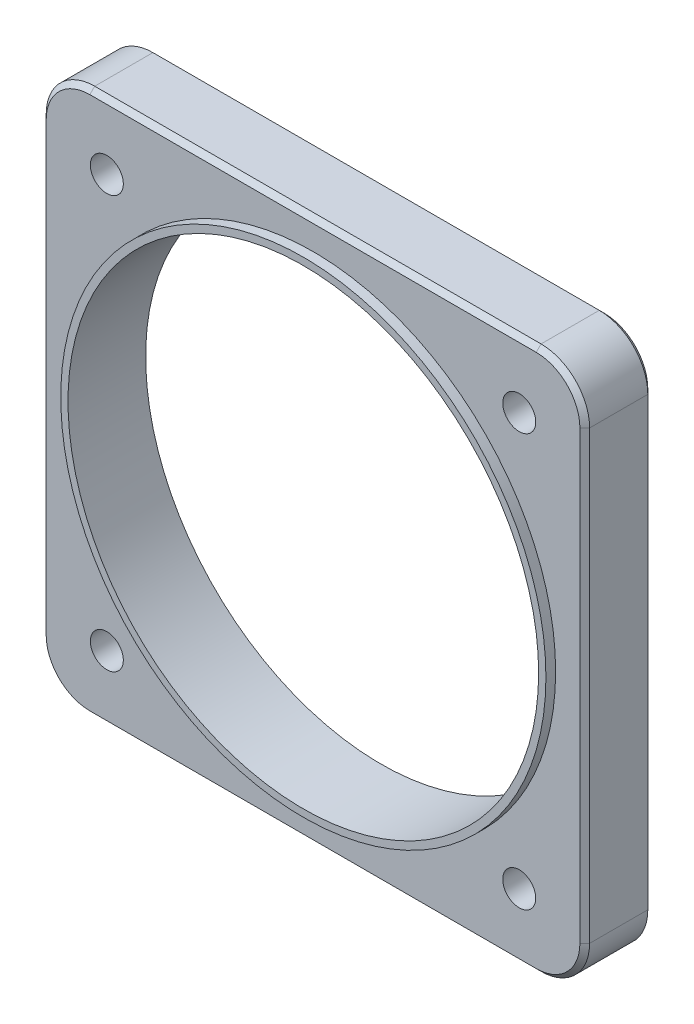
from build123d import *

# Parameters (mm, degrees)
SKETCH1_R           = 48.5
BOSS_EXTRUDE1_DEPTH = 16
SKETCH2_R           = 3.35
CUT_EXTRUDE1_DEPTH  = 81.796039507
M8_TAPPED_HOLE2_D   = 6.8
CUT_EXTRUDE2_START  = -2
SKETCH5_R           = 50
CUT_EXTRUDE2_DEPTH  = 2
CHAMFER1_SIZE       = 1


with BuildPart() as part:
    # Sketch1 → Boss-Extrude1 (new body)
    with BuildSketch(Plane.XY):
        with BuildLine():
            Line((-46, 56), (46, 56))
            ThreePointArc((46, 56), (53.071067812, 53.071067812), (56, 46))
            Line((56, 46), (56, -46))
            ThreePointArc((56, -46), (53.071067812, -53.071067812), (46, -56))
            Line((46, -56), (-46, -56))
            ThreePointArc((-46, -56), (-53.071067812, -53.071067812), (-56, -46))
            Line((-56, -46), (-56, 46))
            ThreePointArc((-56, 46), (-53.071067812, 53.071067812), (-46, 56))
        make_face()
        Circle(SKETCH1_R, mode=Mode.SUBTRACT)
    extrude(amount=BOSS_EXTRUDE1_DEPTH)

    # Sketch2 → Cut-Extrude1 (cut, through all)
    with BuildSketch(Plane.XY.offset(16)):
        with Locations((-42.5, 42.5)):
            Circle(SKETCH2_R)
        with Locations((42.5, 42.5)):
            Circle(SKETCH2_R)
        with Locations((42.5, -42.5)):
            Circle(SKETCH2_R)
        with Locations((-42.5, -42.5)):
            Circle(SKETCH2_R)
    extrude(amount=-CUT_EXTRUDE1_DEPTH, mode=Mode.SUBTRACT)

    # M8 Tapped Hole2 (through all)
    with Locations(Plane.XY.offset(16)):
        with Locations((-42.5, 42.5), (42.5, 42.5), (42.5, -42.5), (-42.5, -42.5)):
            Hole(M8_TAPPED_HOLE2_D / 2)

    # Sketch5 → Cut-Extrude2 (cut)
    with BuildSketch(Plane.XY.offset(16).offset(CUT_EXTRUDE2_START)):
        with BuildLine():
            Line((56, -46), (56, 46))
            ThreePointArc((56, 46), (53.071067812, 53.071067812), (46, 56))
            Line((46, 56), (-46, 56))
            ThreePointArc((-46, 56), (-53.071067812, 53.071067812), (-56, 46))
            Line((-56, 46), (-56, -46))
            ThreePointArc((-56, -46), (-53.071067812, -53.071067812), (-46, -56))
            Line((-46, -56), (46, -56))
            ThreePointArc((46, -56), (53.071067812, -53.071067812), (56, -46))
        make_face()
        Circle(SKETCH5_R, mode=Mode.SUBTRACT)
    extrude(amount=CUT_EXTRUDE2_DEPTH, mode=Mode.SUBTRACT)

    # Chamfer1
    chamfer1_edges = [part.edges().sort_by_distance(p)[0] for p in [
        (56, 0, 0),
        (53.071067812, -53.071067812, 0),
        (0, -56, 0),
        (-53.071067812, -53.071067812, 0),
        (-56, 0, 0),
        (-53.071067812, 53.071067812, 0),
        (0, 56, 0),
        (53.071067812, 53.071067812, 14),
        (56, 0, 14),
        (53.071067812, -53.071067812, 14),
        (0, -56, 14),
        (-53.071067812, -53.071067812, 14),
        (-56, 0, 14),
        (-53.071067812, 53.071067812, 14),
        (0, 56, 14),
        (53.071067812, 53.071067812, 0),
    ]]
    chamfer(chamfer1_edges, length=CHAMFER1_SIZE)


solid = part.part
